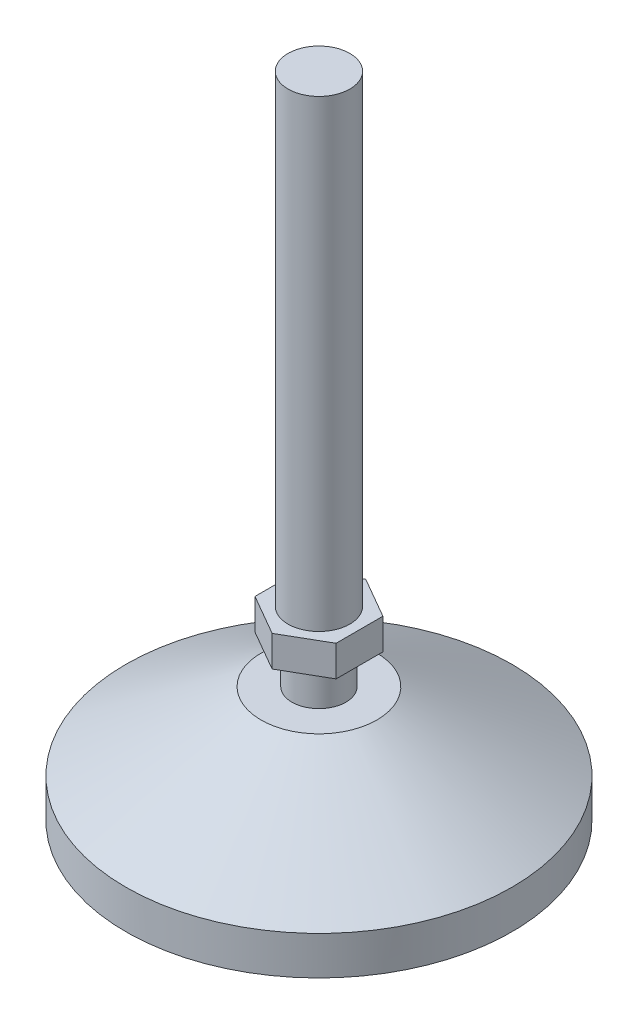
SolidWorks part; units mm, degrees
ref_plane "前视基准面" through (0, 0, 0) normal (0, 0, 1) x (1, 0, 0)
ref_plane "上视基准面" through (0, 0, 0) normal (0, 1, 0) x (1, 0, 0)
ref_plane "右视基准面" through (0, 0, 0) normal (1, 0, 0) x (0, 0, -1)
sketch "草图1" plane through (0, 0, 0) normal (0, 0, 1) x (1, 0, 0)
  line L0 (0, 30) -> (0, 0)
  line L1 (0, 0) -> (50, 0)
  line L2 (50, 0) -> (50, 10)
  line L3 (50, 10) -> (15, 30)
  line L4 (15, 30) -> (0, 30)
  dimension "D1" = 15
  dimension "D2" = 30
  dimension "D3" = 50
  dimension "D4" = 10
revolve "旋转1" add sketch "草图1" angle 360 about L0
sketch "草图2" plane through (0, 30, 0) normal (0, 1, 0) x (1, 0, 0)
  circle A0 centre (0, 0) radius 7
  dimension "D1" = 14
extrude "凸台-拉伸1" add sketch "草图2" along normal blind 10
sketch "草图3" plane through (0, 40, 0) normal (0, 1, 0) x (1, 0, 0)
  line L0 (0, 0) -> (0, 23.0176) construction
  line L1 (0, 12.1244) -> (-10.5, 6.0622)
  line L2 (-10.5, 6.0622) -> (-10.5, -6.0622)
  line L3 (-10.5, -6.0622) -> (0, -12.1244)
  line L4 (0, -12.1244) -> (10.5, -6.0622)
  line L5 (10.5, -6.0622) -> (10.5, 6.0622)
  line L6 (10.5, 6.0622) -> (0, 12.1244)
  circle A0 centre (0, 0) radius 10.5 construction
  dimension "D1" = 21
extrude "凸台-拉伸2" add sketch "草图3" along normal blind 8
sketch "草图4" plane through (0, 48, 0) normal (0, 1, 0) x (1, 0, 0)
  circle A0 centre (0, 0) radius 8
  dimension "D1" = 16
extrude "凸台-拉伸3" add sketch "草图4" along normal blind 120
